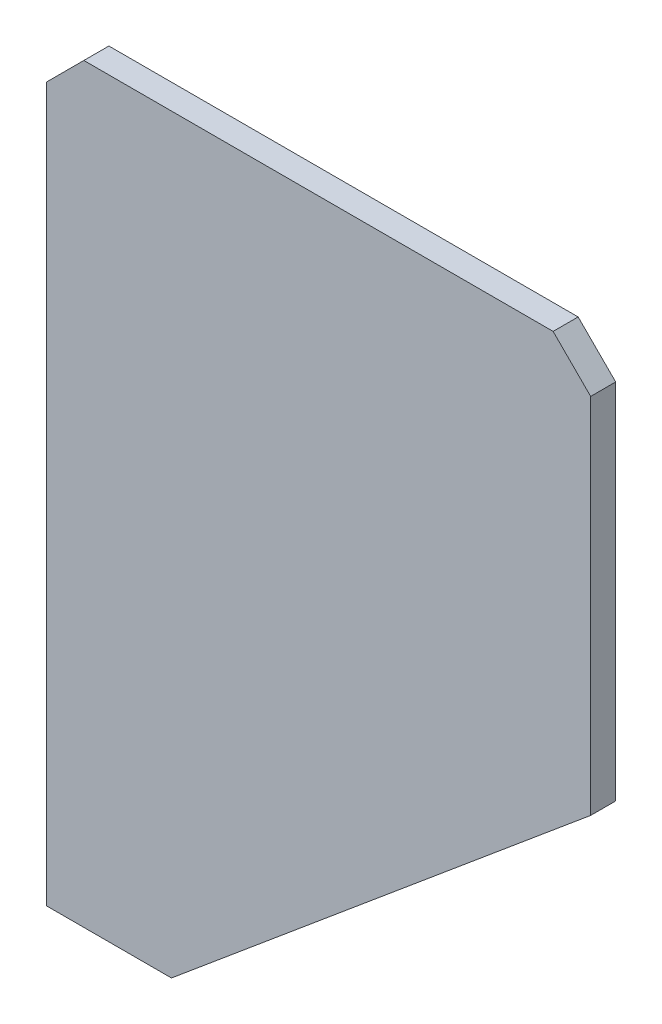
from build123d import *

# Parameters (mm, degrees)
EXTRUDE_1_DEPTH = 2
CHAMFER_1_SIZE  = 3


with BuildPart() as part:
    # 草图1 → 凸台-拉伸1 (new body)
    with BuildSketch(Plane.XY):
        Polygon((0, 0), (43.5, 0), (43.5, -32), (10, -60), (0, -60), align=None)
    extrude(amount=EXTRUDE_1_DEPTH)

    # 倒角1
    chamfer_1_edges = [part.edges().sort_by_distance(p)[0] for p in [
        (0, 0, 1),
        (43.5, 0, 1),
    ]]
    chamfer(chamfer_1_edges, length=CHAMFER_1_SIZE)


solid = part.part
